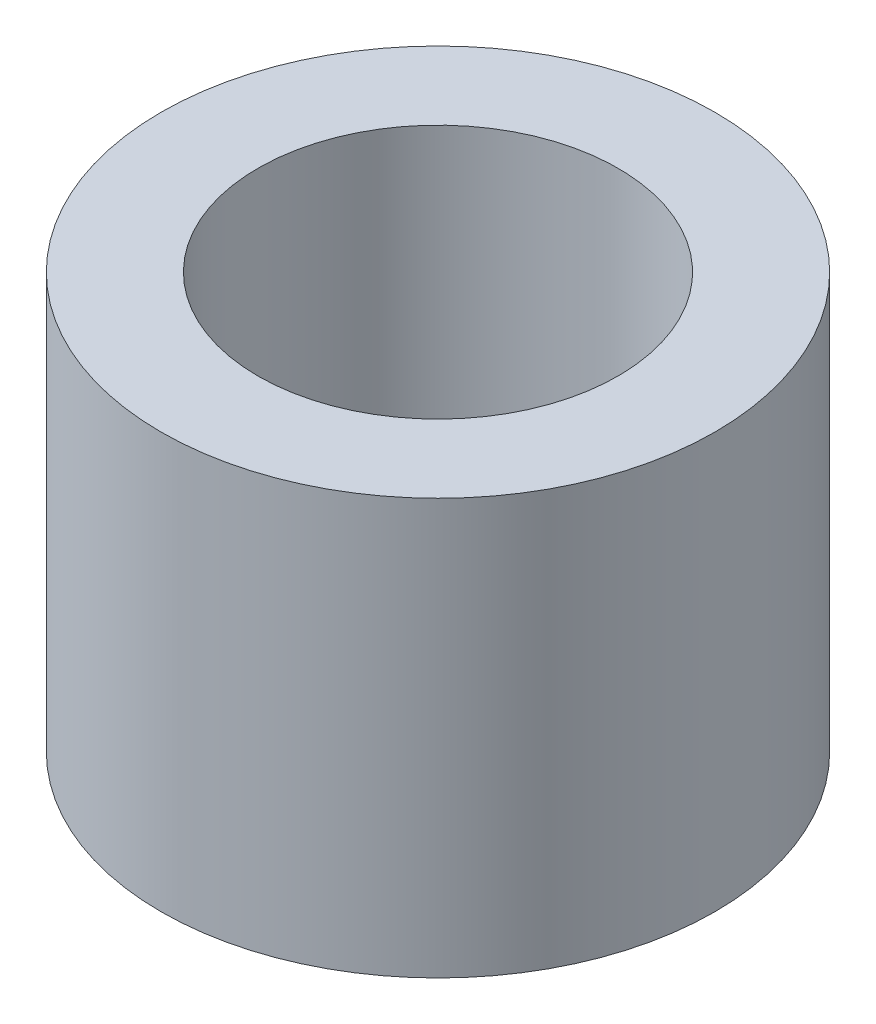
SolidWorks part; units mm, degrees
ref_plane "Front Plane" through (0, 0, 0) normal (0, 0, 1) x (1, 0, 0)
ref_plane "Top Plane" through (0, 0, 0) normal (0, 1, 0) x (1, 0, 0)
ref_plane "Right Plane" through (0, 0, 0) normal (1, 0, 0) x (0, 0, -1)
sketch "Sketch1" plane through (0, 0, 0) normal (0, 1, 0) x (1, 0, 0)
  circle A0 centre (0, 0) radius 2.6
  circle A1 centre (0, 0) radius 4
  dimension "D1" = 5.2
  dimension "D2" = 8
extrude "Boss-Extrude1" add sketch "Sketch1" along normal blind 6
